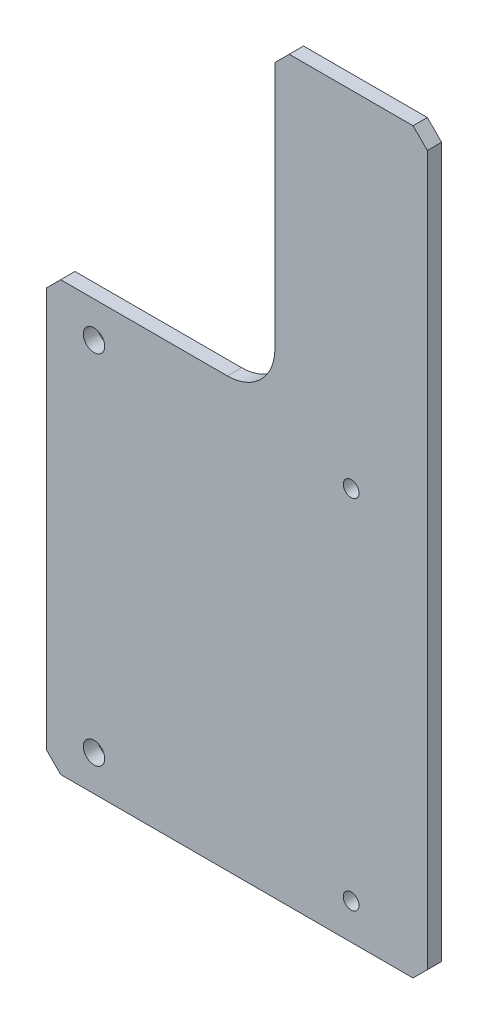
SolidWorks part; units mm, degrees
material "SUS304"
ref_plane "Front Plane" through (0, 0, 0) normal (0, 0, 1) x (1, 0, 0)
ref_plane "Top Plane" through (0, 0, 0) normal (0, 1, 0) x (1, 0, 0)
ref_plane "Right Plane" through (0, 0, 0) normal (1, 0, 0) x (0, 0, -1)
sketch "Sketch1" plane through (0, 0, 0) normal (0, 0, 1) x (1, 0, 0)
  line L1 (0, 0) -> (80, 0)
  line L2 (0, 0) -> (0, 155)
  line L3 (0, 155) -> (80, 155)
  line L4 (80, 0) -> (80, 155)
  dimension "D1" = 155
  dimension "D2" = 80
extrude "Boss-Extrude1" add sketch "Sketch1" along normal blind 3
hole_wizard "M4 Tapped Hole1" positions "Sketch3" profile "Sketch4" tap size "M4" standard "Gb" end condition through all
sketch "Sketch3" plane through (0, 0, 3) normal (0, 0, 1) x (1, 0, 0)
  line L1 (80, 0) -> (80, 155) construction
  line L4 (0, 0) -> (80, 0) construction
  point P0 (64, 82.5)
  point P2 (64, 7.5)
  dimension "D1" = 75
  dimension "D2" = 16
  dimension "D3" = 7.5
sketch "Sketch4" plane through (64, 82.5, 3) normal (1, 0, 0) x (0, -1, 0)
  line L0 (0, 0) -> (0, 3)
  line L1 (0, 3) -> (1.65, 3)
  line L2 (1.65, 3) -> (1.65, 0)
  line L5 (1.65, 0) -> (0, 0)
  line L11 (0, -6.35) -> (0, 107.95) construction
  dimension "通孔螺纹孔钻头直径" = 3.3
  dimension "通孔螺纹孔钻头深度" = 3
cosmetic thread "Hole thread 1" parameters "D2"=4
cosmetic thread "Hole thread 2" parameters "D2"=4
hole_wizard "M4 Clearance Hole1" positions "Sketch6" profile "Sketch7" hole size "M4" standard "Gb" end condition through all
sketch "Sketch6" plane through (0, 0, 3) normal (0, 0, 1) x (1, 0, 0)
  line L0 (64, 82.5) -> (10, 82.5) construction
  line L2 (10, 7.5) -> (64, 7.5) construction
  line L4 (0, 155) -> (0, 0) construction
  point P0 (10, 82.5)
  point P2 (10, 7.5)
  dimension "D1" = 10
sketch "Sketch7" plane through (10, 82.5, 3) normal (1, 0, 0) x (0, -1, 0)
  line L0 (0, 0) -> (0, 3)
  line L1 (0, 3) -> (2.25, 3)
  line L2 (2.25, 3) -> (2.25, 0)
  line L5 (2.25, 0) -> (0, 0)
  line L11 (0, -6.35) -> (0, 107.95) construction
  dimension "通孔孔直径" = 4.5
  dimension "通孔孔深度" = 3
sketch "Sketch8" plane through (0, 0, 3) normal (0, 0, 1) x (1, 0, 0)
  line L0 (80, 155) -> (0, 155) construction
  line L1 (48, 90) -> (0, 90)
  line L2 (48, 90) -> (48, 155)
  line L3 (48, 155) -> (0, 155)
  line L4 (0, 90) -> (0, 155)
  line L5 (80, 0) -> (80, 155) construction
  line L6 (0, 0) -> (80, 0) construction
  line L7 (0, 155) -> (0, 0) construction
  dimension "D1" = 32
  dimension "D2" = 90
extrude "Cut-Extrude1" cut sketch "Sketch8" against normal through all
chamfer "Chamfer1" distance 3 angle 45 5 edges at (0, 0, 1.5) (80, 0, 1.5) (80, 155, 1.5) (48, 155, 1.5) (0, 90, 1.5)
fillet "Fillet1" radius 10 1 edges at (48, 90, 1.5)
